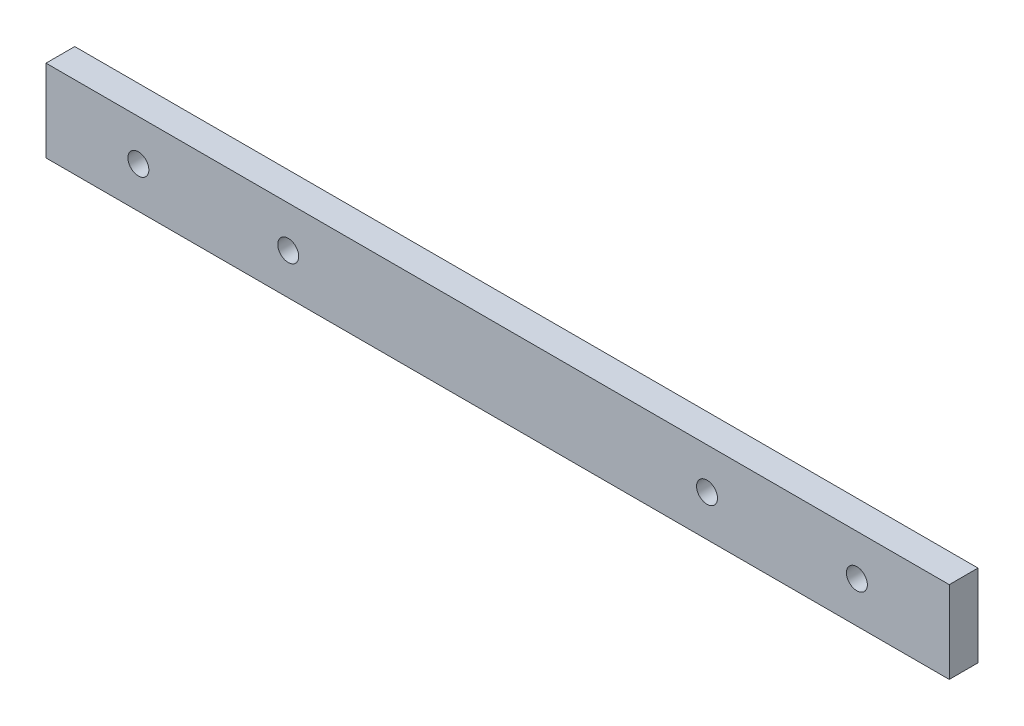
from build123d import *

# Parameters (mm, degrees)
SKETCH_1_W              = 440
SKETCH_1_H              = 40
EXTRUDE_1_DEPTH         = 14
HOLE_WIZARD_M12_1_D     = 10.2
HOLE_WIZARD_M12_1_DEPTH = 29.25
HOLE_WIZARD_M12_1_TIP   = 3.064389157


with BuildPart() as part:
    # 草图1 → 凸台-拉伸1 (new body)
    with BuildSketch(Plane.XY):
        with Locations((220, 20)):
            Rectangle(SKETCH_1_W, SKETCH_1_H)
    extrude(amount=EXTRUDE_1_DEPTH)

    # M12 螺纹孔1
    with Locations(Plane(origin=(45, 20, 14), x_dir=(1, 0, 0), z_dir=(0, 0, 1))):
        with Locations((0, 0), (73, 0), (350, 0), (277, 0)):
            Hole(HOLE_WIZARD_M12_1_D / 2, depth=HOLE_WIZARD_M12_1_DEPTH)
            with Locations((0, 0, -(HOLE_WIZARD_M12_1_DEPTH + HOLE_WIZARD_M12_1_TIP / 2))):  # 118° drill point
                Cone(0, HOLE_WIZARD_M12_1_D / 2, HOLE_WIZARD_M12_1_TIP, mode=Mode.SUBTRACT)


solid = part.part
